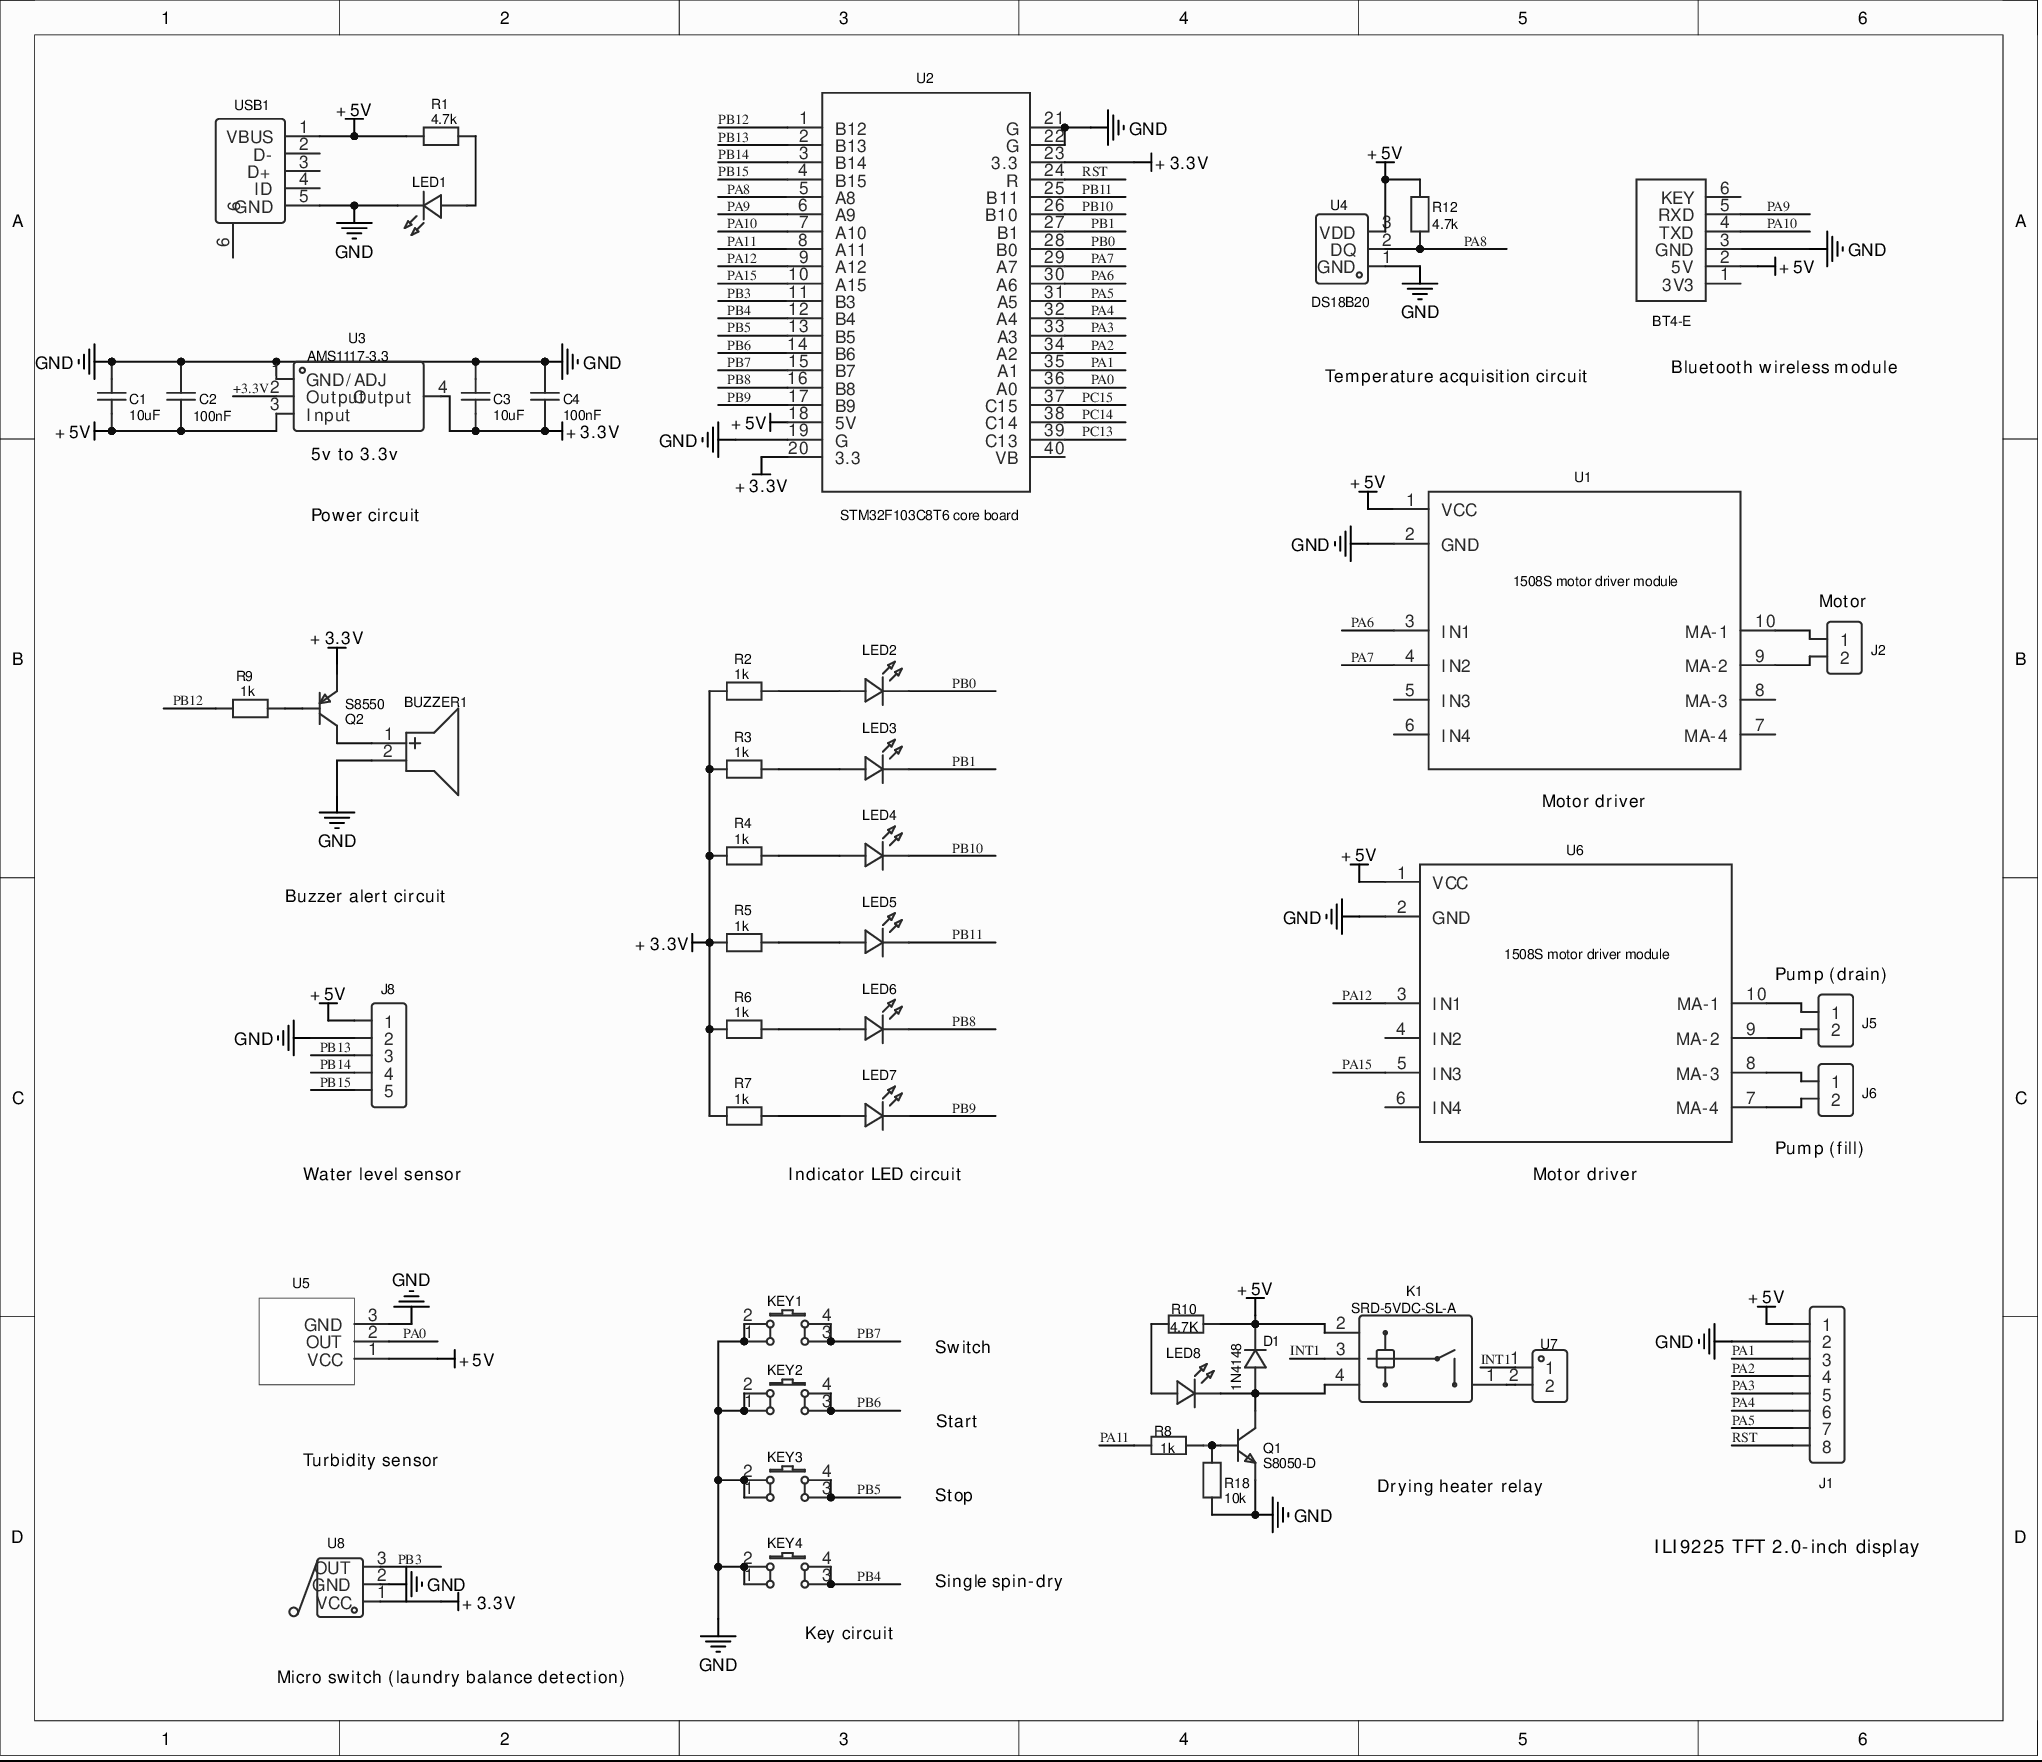
[diagram p0: MISC82193-4.SchDoc]
# Altium project MISC82193-7.PrjPcb
1 sheet, 48 parts. Net scope: global (net labels, ports and power ports of the same name join across sheets).
Board file: MISC82193.PcbDoc

## Sheet MISC82193-4.SchDoc
size 298 x 257 mm

### Parts
BT4-E  NO  [HDR1X6]  (value not drawn)
BUZZER1  5V  [PIN2]  (value not drawn)
C1  10uF  [C0805]
C2  100nF  [C0805]
C3  10uF  [C0805]
C4  100nF  [C0805]
D1  1N4148  [DO-35]
J1  HDR-M-2.54_1x8  [HDR1X8]  (value not drawn)
J2  HDR-M-2.54_1x2  [HDR1X2]  (value not drawn)
J5  HDR-M-2.54_1x2  [HDR1X2]  (value not drawn)
J6  HDR-M-2.54_1x2  [HDR1X2]  (value not drawn)
J8  HDR-M-2.54_1x5  [HDR1X5]  (value not drawn)
K1  SRD-5VDC-SL-A  [012-1HW_BK]
KEY1  K4-6×6_TH  [四脚轻触开关]  (value not drawn)
KEY2  K4-6×6_TH  [四脚轻触开关]  (value not drawn)
KEY3  K4-6×6_TH  [四脚轻触开关]  (value not drawn)
KEY4  K4-6×6_TH  [四脚轻触开关]  (value not drawn)
LED1  LED-TH-3mm_R  [LED-1]  (value not drawn)
LED2  LED-0603_R  [LED-1]  (value not drawn)
LED3  LED-0603_R  [LED-1]  (value not drawn)
LED4  LED-0603_R  [LED-1]  (value not drawn)
LED5  LED-0603_R  [LED-1]  (value not drawn)
LED6  LED-0603_R  [LED-1]  (value not drawn)
LED7  LED-0603_R  [LED-1]  (value not drawn)
LED8  LED-TH-3mm_R  [LED-1]  (value not drawn)
Q1  S8050-D  [TO-92A]
Q2  S8550  [TO-92A]
R1  4.7k  [AXIAL-0.3]
R2  1k  [AXIAL-0.3]
R3  1k  [AXIAL-0.3]
R4  1k  [AXIAL-0.3]
R5  1k  [AXIAL-0.3]
R6  1k  [AXIAL-0.3]
R7  1k  [AXIAL-0.3]
R8  1k  [AXIAL-0.3]
R9  1k  [AXIAL-0.3]
R10  4.7K  [AXIAL-0.3]
R12  4.7k  [AXIAL-0.3]
R18  10k  [AXIAL-0.3]
U1  1508S motor driver module  [DIANJIQUDONG]
U2  STM32F103C8T6 core board  [STM32核心板]
U3  AMS1117-3.3  [AMS1117-3.3]
U4  DS18B20  [DS18B20]
U5  NO  [HDR1X3]  (value not drawn)
U6  1508S motor driver module  [DIANJIQUDONG]
U7  Connect watering pump  [HDR1X2]  (value not drawn)
U8  NO  [xianwei]  (value not drawn)
USB1  MICRO5.9MMUSB  [MICRO-USB-SMD_5P-P0.65-H-F_MICRO5.9MMUSB]  (value not drawn)

### Nets
+3.3V: C3.2 C4.1 Q2.1(E) R2.1 R3.1 R4.1 R5.1 R6.1 R7.1 U2.20(3.3) U2.23(3.3) U3.2(Output) U3.4(Output) U8.1(VCC)
+5V: BT4-E.2(5V) C1.1 C2.1 D1.1(C) J1.1 J8.1 K1.2 R1.1 R10.2 R12.2 U1.1(VCC) U2.18(5V) U3.3(Input) U4.3(VDD) U5.1(VCC) U6.1(VCC) USB1.1(VBUS)
GND: BT4-E.3(GND) BUZZER1.2(-) C1.2 C2.2 C3.1 C4.2 J1.2 J8.2 KEY1.1 KEY1.2 KEY2.1 KEY2.2 KEY3.1 KEY3.2 KEY4.1 KEY4.2 LED1.2 Q1.1(E) R18.1 U1.2(GND) U2.19(G) U2.21(G) U2.22(G) U3.1(GND/ADJ) U4.1(GND) U5.3(GND) U6.2(GND) U8.2(GND) USB1.5(GND)
INT1: K1.3 U7.1
PA0: U2.36(A0) U5.2(OUT)
PA1: J1.3 U2.35(A1)
PA2: J1.4 U2.34(A2)
PA3: J1.5 U2.33(A3)
PA4: J1.6 U2.32(A4)
PA5: J1.7 U2.31(A5)
PA6: U1.3(IN1) U2.30(A6)
PA7: U1.4(IN2) U2.29(A7)
PA8: R12.1 U2.5(A8) U4.2(DQ)
PA9: BT4-E.5(RXD) U2.6(A9)
PA10: BT4-E.4(TXD) U2.7(A10)
PA11: R8.1 U2.8(A11)
PA12: U2.9(A12) U6.3(IN1)
PA15: U2.10(A15) U6.5(IN3)
PB0: LED2.2 U2.28(B0)
PB1: LED3.2 U2.27(B1)
PB3: U2.11(B3) U8.3(OUT)
PB4: KEY4.3 KEY4.4 U2.12(B4)
PB5: KEY3.3 KEY3.4 U2.13(B5)
PB6: KEY2.3 KEY2.4 U2.14(B6)
PB7: KEY1.3 KEY1.4 U2.15(B7)
PB8: LED6.2 U2.16(B8)
PB9: LED7.2 U2.17(B9)
PB10: LED4.2 U2.26(B10)
PB11: LED5.2 U2.25(B11)
PB12: R9.1 U2.1(B12)
PB13: J8.3 U2.2(B13)
PB14: J8.4 U2.3(B14)
PB15: J8.5 U2.4(B15)
PC13: U2.39(C13)
PC14: U2.38(C14)
PC15: U2.37(C15)
RST: J1.8 U2.24(R)
NetBUZZER1_1: BUZZER1.1(+) Q2.3(C)
NetD1_2: D1.2(A) K1.4 LED8.2 Q1.3(C)
NetJ2_1: J2.1 U1.10(MA-1)
NetJ2_2: J2.2 U1.9(MA-2)
NetJ5_1: J5.1 U6.10(MA-1)
NetJ5_2: J5.2 U6.9(MA-2)
NetJ6_1: J6.1 U6.8(MA-3)
NetJ6_2: J6.2 U6.7(MA-4)
NetK1_1: K1.1 U7.2
NetLED1_1: LED1.1 R1.2
NetLED2_1: LED2.1 R2.2
NetLED3_1: LED3.1 R3.2
NetLED4_1: LED4.1 R4.2
NetLED5_1: LED5.1 R5.2
NetLED6_1: LED6.1 R6.2
NetLED7_1: LED7.1 R7.2
NetLED8_1: LED8.1 R10.1
NetQ1_2: Q1.2(B) R8.2 R18.2
NetQ2_2: Q2.2(B) R9.2

Not connected (* = marked no-connect by the designer): BT4-E 1(3V3)* 6(KEY)*; U1 5(IN3)* 6(IN4)* 7(MA-4)* 8(MA-3)*; U2 40(VB)*; U6 4(IN2)* 6(IN4)*; USB1 2(D-)* 3(D+)* 4(ID)* 6*

### Notes on the sheet
- Temperature acquisition circuit
- Bluetooth wireless module
- (near U3) 5v to 3.3v
- Power circuit
- (near J2) Motor
- Motor driver
- Buzzer alert circuit
- Pump (drain)
- Water level sensor
- Indicator LED circuit
- (near U6) Motor driver
- Pump (fill)
- Switch
- Start
- Turbidity sensor
- Stop
- Drying heater relay
- Single spin-dry
- ILI9225 TFT 2.0-inch display
- (near U8) Micro switch (laundry balance detection)
- (near KEY4) Key circuit

### Library data of the parts
BT4-E = NO: Contributor: Aries-Vino; spicePre: U; spiceSymbolName: BT04-E Bluetooth module COPY
BUZZER1 = 5V: Manufacturer: INGHAi; Manufacturer Part: GMD12095YB-5V2400; Contributor: LCSC; SMT Type: Extend; Supplier: LCSC; Supplier Part: C252941; JLCPCB SMD: Yes; spicePre: B; spiceSymbolName: GMD12095YB-5V2400
C1 C3 = 10uF: Manufacturer: HEC(Holy Stone Enterprise); Manufacturer Part: C0805X104K101T; nameAlias: Capacitance; Contributor: LCSC; Supplier: LCSC; Supplier Part: C485772; spicePre: C; spiceSymbolName: C0805X104K101T_C485772
C2 C4 = 100nF: Manufacturer: HEC(Holy Stone Enterprise); Manufacturer Part: C0805X104K101T; nameAlias: Capacitance; Contributor: LCSC; Supplier: LCSC; Supplier Part: C485772; spicePre: C; spiceSymbolName: C0805X104K101T_C485772
D1 = 1N4148: Manufacturer: STARSEA; Supplier: LCSC; Manufacturer Part: 1N4148; Supplier Part: C85057; spicePre: D; spiceSymbolName: 1N4148-C85057
J1 = HDR-M-2.54_1x8: Contributor: LCEDA_Lib; Supplier Part: C190820; Supplier: LCSC; spicePre: J; spiceSymbolName: HDR-M-2.54_1x8
J2 J5 J6 = HDR-M-2.54_1x2: Contributor: LCEDA_Lib; Supplier Part: C124375; Supplier: LCSC; spicePre: J; spiceSymbolName: HDR-M-2.54_1x2
J8 = HDR-M-2.54_1x5: Contributor: LCEDA_Lib; Supplier Part: C358687; Supplier: LCSC; spicePre: J; spiceSymbolName: HDR-M-2.54_1x5
K1 = SRD-5VDC-SL-A: Manufacturer: Ningbo Songle Relay; Contributor: LCSC; SMT Type: Extend; Supplier: LCSC; Supplier Part: C140615; Manufacturer Part: SRD-5VDC-SL-A; JLCPCB SMD: Yes; spicePre: K; spiceSymbolName: SRD-5VDC-SL-A
KEY1-KEY4 = K4-6×6_TH: Manufacturer: 韩国韩荣; Manufacturer Part: K2-1102DP-E4SW-04; Contributor: LCEDA_Lib; Supplier: LCSC; Supplier Part: C136684; spicePre: K; spiceSymbolName: K4-6×6_TH
LED1 LED8 = LED-TH-3mm_R: Manufacturer: EVERLIGHT(台湾亿光); Manufacturer Part: 204-10SDRD/S530-A3-L; Contributor: LCEDA_Lib; Supplier Part: C84774; Supplier: LCSC; spicePre: L; spiceSymbolName: LED-TH-3mm_R
LED2-LED7 = LED-0603_R: Manufacturer: EVERLIGHT(台湾亿光); Manufacturer Part: 19-217/R6C-AL1M2VY/3T; Contributor: LCEDA_01; Supplier Part: C72044; Supplier: LCSC; spicePre: L; spiceSymbolName: LED-0603_R
Q1 = S8050-D: Manufacturer: Foshan Blue Rocket Elec; Contributor: LCSC; Supplier: LCSC; Supplier Part: C305417; Manufacturer Part: S8050-D; JLCPCB Part Class: Extended Part; spicePre: Q; spiceSymbolName: S8050-D
Q2 = S8550: Manufacturer: LGE; Contributor: LCSC; SMT Type: Extend; Supplier: LCSC; Supplier Part: C717454; Manufacturer Part: S8550; JLCPCB SMD: Yes; spicePre: Q; spiceSymbolName: S8550_C717454
R1 R12 = 4.7k: nameAlias: Value(Ω); Contributor: LCEDA_Lib; spicePre: R
  R1: spiceSymbolName: R_0805_EU
  R12: spiceSymbolName: R_AXIAL-0.3_EU
R2-R9 = 1k: nameAlias: Value(Ω); Contributor: LCEDA_Lib; spicePre: R
  R2-R7: spiceSymbolName: R_0603_EU
  R8 R9: spiceSymbolName: R_AXIAL-0.3_EU
R10 = 4.7K: nameAlias: Value(Ω); Contributor: LCEDA_Lib; spicePre: R; spiceSymbolName: R_AXIAL-0.3_EU
R18 = 10k: nameAlias: Value(Ω); Contributor: LCEDA_Lib; spicePre: R; spiceSymbolName: R_AXIAL-0.3_EU
U1 U6 = 电机驱动1508S模块: Contributor: Asuka_Whw; spicePre: U; spiceSymbolName: Small motor driver
U2 = STM32F103C8T6核心板: Contributor: Ahren-5; Convert to PCB: Yes; Add into BOM: Yes; spicePre: U; spiceSymbolName: STM32F103C8T6 core board
U3 = AMS1117-3.3: Manufacturer: KEXIN; Contributor: LCSC; SMT Type: Extend; Supplier: LCSC; Supplier Part: C369933; Manufacturer Part: AMS1117-3.3; JLCPCB SMD: Yes; spicePre: U; spiceSymbolName: AMS1117-3.3_C369933
U4 = DS18B20: Manufacturer: Youtai Semiconductor Co., Ltd.; Contributor: LCSC; SMT Type: Extend; Supplier: LCSC; Supplier Part: C376006; Manufacturer Part: DS18B20; JLCPCB SMD: Yes; spicePre: U; spiceSymbolName: DS18B20
U5 = NO: Contributor: DuTesz; spicePre: U; spiceSymbolName: TS-300B_____
U7 = 接浇水水泵: Manufacturer: Cixi Kefa Elec; Manufacturer Part: KF301-5.0-2P; Contributor: LCSC; SMT Type: Extend; Supplier: LCSC; Supplier Part: C474881; JLCPCB SMD: Yes; spicePre: U; spiceSymbolName: KF301-5.0-2P
U8 = NO: Manufacturer: null; Manufacturer Part: 2.54排针1x3; Contributor: r980ah; Supplier Part: C9900014022; JLCPCB Part Class: Extended Part; spicePre: U; spiceSymbolName: Limit switch module
USB1 = MICRO5.9MMUSB: Manufacturer: SHOU HAN; Contributor: LCSC; Supplier: LCSC; Supplier Part: C393940; Manufacturer Part: MICRO5.9mmusb; spicePre: U; spiceSymbolName: MICRO5.9MMUSB